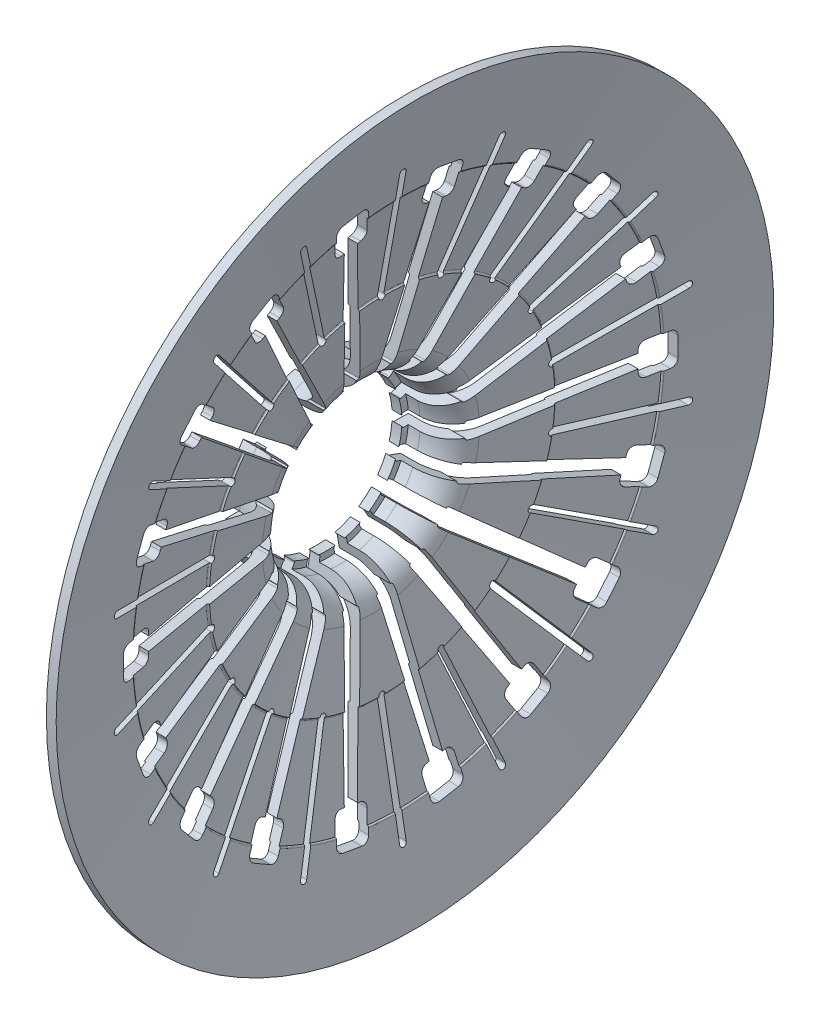
SolidWorks part; units mm, degrees
ref_plane "Front Plane" through (0, 0, 0) normal (0, 0, 1) x (1, 0, 0)
ref_plane "Top Plane" through (0, 0, 0) normal (0, 1, 0) x (1, 0, 0)
ref_plane "Right Plane" through (0, 0, 0) normal (1, 0, 0) x (0, 0, -1)
other "Configuration Table"
sketch "Sketch2" plane through (0, 0, 0) normal (0, 0, 1) x (1, 0, 0)
  line L0 (1418.6702, 525.6363) -> (1415.6702, 525.6363)
  line L1 (1418.6702, 415.6363) -> (1388.6702, 415.6363) construction
  line L2 (1388.6702, 415.6363) -> (1388.6702, 443.6363)
  line L3 (1415.6702, 525.6363) -> (1410.6453, 497.1385)
  line L4 (1418.6702, 415.6363) -> (1418.6702, 525.6363) construction
  line L5 (1388.6702, 443.6363) -> (1392.8204, 443.6363)
  line L6 (1418.6702, 525.6363) -> (1413.6453, 497.1385)
  line L7 (1325.0417, 415.6363) -> (1423.6069, 415.6363) construction
  line L8 (1388.6702, 415.6363) -> (1391.6702, 415.6363)
  line L9 (1391.6702, 440.6363) -> (1395.2915, 440.6363)
  line L10 (1391.6702, 415.6363) -> (1391.6702, 440.6363)
  line L11 (1410.1533, 496.7273) -> (1405.181, 469.169)
  line L12 (1408.6104, 468.5841) -> (1405.1395, 448.8998)
  line L13 (1405.6104, 468.5841) -> (1402.6685, 451.8998)
  line L30 (1413.1533, 496.7273) -> (1408.181, 469.169)
  arc A0 (1392.8204, 443.6363) -> (1402.6685, 451.8998) centre (1392.8204, 453.6363) ccw
  arc A1 (1395.2915, 440.6363) -> (1405.1395, 448.8998) centre (1395.2915, 450.6363) ccw
  arc A10 (1413.1533, 496.7273) -> (1413.6453, 497.1385) centre (1413.1533, 497.2273) ccw
  arc A11 (1405.181, 469.169) -> (1405.6104, 468.5841) centre (1405.6731, 469.0802) ccw
  arc A12 (1408.181, 469.169) -> (1408.6104, 468.5841) centre (1408.6731, 469.0802) ccw
  arc A13 (1410.1533, 496.7273) -> (1410.6453, 497.1385) centre (1410.1533, 497.2273) ccw
  dimension "D5" = 10
  dimension "D6" = 10
  dimension "D2" = 30
  dimension "D3" = 110
  dimension "D4" = 3
revolve "Revolve1" add sketch "Sketch2" angle 360 about L7
sketch "Sketch8" plane through (0, 0, 0) normal (1, 0, 0) x (0, 0, -1)
  line L0 (0, 525.6363) -> (0, 504.6363) construction
  line L1 (0, 504.6363) -> (0, 468.6363) construction
  line L2 (30.4398, 499.269) -> (18.1271, 465.44) construction
  line L3 (1, 504.6363) -> (1, 468.6363)
  line L4 (-1, 504.6363) -> (-1, 468.6363)
  line L5 (31.3795, 498.9269) -> (19.0668, 465.098)
  line L6 (29.5001, 499.611) -> (17.1874, 465.7821)
  line L7 (57.2081, 483.8143) -> (34.0677, 456.2367) construction
  line L8 (57.9741, 483.1715) -> (34.8338, 455.5939)
  line L9 (56.4421, 484.4571) -> (33.3017, 456.8795)
  line L10 (77.0763, 460.1363) -> (45.8993, 442.1363) construction
  line L11 (77.5763, 459.2703) -> (46.3993, 441.2703)
  line L12 (76.5763, 461.0023) -> (45.3993, 443.0023)
  line L13 (87.6479, 431.091) -> (52.1948, 424.8397) construction
  line L14 (87.8215, 430.1062) -> (52.3685, 423.8549)
  line L15 (87.4742, 432.0758) -> (52.0212, 425.8245)
  line L16 (87.6479, 400.1816) -> (52.1948, 406.433) construction
  line L17 (87.4742, 399.1968) -> (52.0212, 405.4482)
  line L18 (87.8215, 401.1664) -> (52.3685, 407.4178)
  line L19 (77.0763, 371.1363) -> (45.8993, 389.1363) construction
  line L20 (76.5763, 370.2703) -> (45.3993, 388.2703)
  line L21 (77.5763, 372.0023) -> (46.3993, 390.0023)
  line L22 (57.2081, 347.4584) -> (34.0677, 375.036) construction
  line L23 (56.4421, 346.8156) -> (33.3017, 374.3932)
  line L24 (57.9741, 348.1012) -> (34.8338, 375.6788)
  line L25 (30.4398, 332.0037) -> (18.1271, 365.8326) construction
  line L26 (29.5001, 331.6617) -> (17.1874, 365.4906)
  line L27 (31.3795, 332.3457) -> (19.0668, 366.1746)
  line L28 (0, 326.6363) -> (0, 362.6363) construction
  line L29 (-1, 326.6363) -> (-1, 362.6363)
  line L30 (1, 326.6363) -> (1, 362.6363)
  line L31 (-30.4398, 332.0037) -> (-18.1271, 365.8326) construction
  line L32 (-31.3795, 332.3457) -> (-19.0668, 366.1746)
  line L33 (-29.5001, 331.6617) -> (-17.1874, 365.4906)
  line L34 (-57.2081, 347.4584) -> (-34.0677, 375.036) construction
  line L35 (-57.9741, 348.1012) -> (-34.8338, 375.6788)
  line L36 (-56.4421, 346.8156) -> (-33.3017, 374.3932)
  line L37 (-77.0763, 371.1363) -> (-45.8993, 389.1363) construction
  line L38 (-77.5763, 372.0023) -> (-46.3993, 390.0023)
  line L39 (-76.5763, 370.2703) -> (-45.3993, 388.2703)
  line L40 (-87.6479, 400.1816) -> (-52.1948, 406.433) construction
  line L41 (-87.8215, 401.1664) -> (-52.3685, 407.4178)
  line L42 (-87.4742, 399.1968) -> (-52.0212, 405.4482)
  line L43 (-87.6479, 431.091) -> (-52.1948, 424.8397) construction
  line L44 (-87.4742, 432.0758) -> (-52.0212, 425.8245)
  line L45 (-87.8215, 430.1062) -> (-52.3685, 423.8549)
  line L46 (-77.0763, 460.1363) -> (-45.8993, 442.1363) construction
  line L47 (-76.5763, 461.0023) -> (-45.3993, 443.0023)
  line L48 (-77.5763, 459.2703) -> (-46.3993, 441.2703)
  line L49 (-57.2081, 483.8143) -> (-34.0677, 456.2367) construction
  line L50 (-56.4421, 484.4571) -> (-33.3017, 456.8795)
  line L51 (-57.9741, 483.1715) -> (-34.8338, 455.5939)
  line L52 (-30.4398, 499.269) -> (-18.1271, 465.44) construction
  line L53 (-29.5001, 499.611) -> (-17.1874, 465.7821)
  line L54 (-31.3795, 498.9269) -> (-19.0668, 465.098)
  circle A0 centre (0, 415.6363) radius 110 construction
  arc A1 (1, 504.6363) -> (-1, 504.6363) centre (0, 504.6363) ccw
  arc A2 (-1, 468.6363) -> (1, 468.6363) centre (0, 468.6363) ccw
  arc A3 (31.3795, 498.9269) -> (29.5001, 499.611) centre (30.4398, 499.269) ccw
  arc A4 (17.1874, 465.7821) -> (19.0668, 465.098) centre (18.1271, 465.44) ccw
  arc A5 (57.9741, 483.1715) -> (56.4421, 484.4571) centre (57.2081, 483.8143) ccw
  arc A6 (33.3017, 456.8795) -> (34.8338, 455.5939) centre (34.0677, 456.2367) ccw
  arc A7 (77.5763, 459.2703) -> (76.5763, 461.0023) centre (77.0763, 460.1363) ccw
  arc A8 (45.3993, 443.0023) -> (46.3993, 441.2703) centre (45.8993, 442.1363) ccw
  arc A9 (87.8215, 430.1062) -> (87.4742, 432.0758) centre (87.6479, 431.091) ccw
  arc A10 (52.0212, 425.8245) -> (52.3685, 423.8549) centre (52.1948, 424.8397) ccw
  arc A11 (87.4742, 399.1968) -> (87.8215, 401.1664) centre (87.6479, 400.1816) ccw
  arc A12 (52.3685, 407.4178) -> (52.0212, 405.4482) centre (52.1948, 406.433) ccw
  arc A13 (76.5763, 370.2703) -> (77.5763, 372.0023) centre (77.0763, 371.1363) ccw
  arc A14 (46.3993, 390.0023) -> (45.3993, 388.2703) centre (45.8993, 389.1363) ccw
  arc A15 (56.4421, 346.8156) -> (57.9741, 348.1012) centre (57.2081, 347.4584) ccw
  arc A16 (34.8338, 375.6788) -> (33.3017, 374.3932) centre (34.0677, 375.036) ccw
  arc A17 (29.5001, 331.6617) -> (31.3795, 332.3457) centre (30.4398, 332.0037) ccw
  arc A18 (19.0668, 366.1746) -> (17.1874, 365.4906) centre (18.1271, 365.8326) ccw
  arc A19 (-1, 326.6363) -> (1, 326.6363) centre (0, 326.6363) ccw
  arc A20 (1, 362.6363) -> (-1, 362.6363) centre (0, 362.6363) ccw
  arc A21 (-31.3795, 332.3457) -> (-29.5001, 331.6617) centre (-30.4398, 332.0037) ccw
  arc A22 (-17.1874, 365.4906) -> (-19.0668, 366.1746) centre (-18.1271, 365.8326) ccw
  arc A23 (-57.9741, 348.1012) -> (-56.4421, 346.8156) centre (-57.2081, 347.4584) ccw
  arc A24 (-33.3017, 374.3932) -> (-34.8338, 375.6788) centre (-34.0677, 375.036) ccw
  arc A25 (-77.5763, 372.0023) -> (-76.5763, 370.2703) centre (-77.0763, 371.1363) ccw
  arc A26 (-45.3993, 388.2703) -> (-46.3993, 390.0023) centre (-45.8993, 389.1363) ccw
  arc A27 (-87.8215, 401.1664) -> (-87.4742, 399.1968) centre (-87.6479, 400.1816) ccw
  arc A28 (-52.0212, 405.4482) -> (-52.3685, 407.4178) centre (-52.1948, 406.433) ccw
  arc A29 (-87.4742, 432.0758) -> (-87.8215, 430.1062) centre (-87.6479, 431.091) ccw
  arc A30 (-52.3685, 423.8549) -> (-52.0212, 425.8245) centre (-52.1948, 424.8397) ccw
  arc A31 (-76.5763, 461.0023) -> (-77.5763, 459.2703) centre (-77.0763, 460.1363) ccw
  arc A32 (-46.3993, 441.2703) -> (-45.3993, 443.0023) centre (-45.8993, 442.1363) ccw
  arc A33 (-56.4421, 484.4571) -> (-57.9741, 483.1715) centre (-57.2081, 483.8143) ccw
  arc A34 (-34.8338, 455.5939) -> (-33.3017, 456.8795) centre (-34.0677, 456.2367) ccw
  arc A35 (-29.5001, 499.611) -> (-31.3795, 498.9269) centre (-30.4398, 499.269) ccw
  arc A36 (-19.0668, 465.098) -> (-17.1874, 465.7821) centre (-18.1271, 465.44) ccw
  point P9 (0, 486.6363)
  point P17 (24.2834, 482.3545)
  point P24 (45.6379, 470.0255)
  point P31 (61.4878, 451.1363)
  point P38 (69.9214, 427.9653)
  point P45 (69.9214, 403.3073)
  point P52 (61.4878, 380.1363)
  point P59 (45.6379, 361.2472)
  point P66 (24.2834, 348.9181)
  point P73 (0, 344.6363)
  point P80 (-24.2834, 348.9181)
  point P87 (-45.6379, 361.2472)
  point P94 (-61.4878, 380.1363)
  point P101 (-69.9214, 403.3073)
  point P108 (-69.9214, 427.9653)
  point P115 (-61.4878, 451.1363)
  point P122 (-45.6379, 470.0255)
  point P129 (-24.2834, 482.3545)
  point P134 (0, 415.6363)
  dimension "D1" = 18
extrude "Cut-Extrude3" cut sketch "Sketch8" along normal blind 1469.5
sketch "Sketch9" plane through (1388.6702, 0, 0) normal (-1, 0, 0) x (0, 0, 1)
  line L0 (-7.2421, 444.8221) -> (-7.1791, 444.8333)
  line L1 (-3.1768, 445.539) -> (-3.2398, 445.5279)
  line L6 (-17.7214, 498.8356) -> (-14.767, 499.3565)
  line L7 (-15.0632, 489.15) -> (-15.985, 488.9875)
  line L8 (-18.3019, 490.6098) -> (-19.3438, 496.5186)
  line L9 (-10.0761, 490.0294) -> (-10.9932, 489.8677)
  line L10 (-8.4538, 492.3463) -> (-9.4957, 498.2551)
  line L11 (-2.1028, 439.0794) -> (-3.2398, 445.5279)
  line L12 (-6.042, 438.3848) -> (-7.1791, 444.8333)
  line L19 (-10.9932, 489.8677) -> (-2.7712, 446.1182)
  line L20 (-15.0632, 489.15) -> (-7.8213, 445.2277)
  line L21 (-11.8126, 499.8774) -> (-14.767, 499.3565)
  arc A0 (-2.54, 438.4956) -> (-5.4315, 437.9858) centre (0, 415.6363) ccw
  arc A4 (-17.7214, 498.8356) -> (-19.3438, 496.5186) centre (-17.3741, 496.8659) ccw
  arc A5 (-18.3019, 490.6098) -> (-15.985, 488.9875) centre (-16.3323, 490.9571) ccw
  arc A6 (-9.4957, 498.2551) -> (-11.8126, 499.8774) centre (-11.4653, 497.9078) ccw
  arc A7 (-10.0761, 490.0294) -> (-8.4538, 492.3463) centre (-10.4234, 491.999) ccw
  arc A8 (-2.54, 438.4956) -> (-2.1028, 439.0794) centre (-2.5952, 438.9926) ccw
  arc A9 (-6.042, 438.3848) -> (-5.4315, 437.9858) centre (-5.5496, 438.4716) ccw
  arc A10 (-3.1768, 445.539) -> (-2.7712, 446.1182) centre (-3.2636, 446.0314) ccw
  arc A11 (-7.8213, 445.2277) -> (-7.2421, 444.8221) centre (-7.3289, 445.3145) ccw
extrude "Cut-Extrude4" cut sketch "Sketch9" against normal through all
sketch "Sketch10" plane through (1388.6702, 0, 0) normal (-1, 0, 0) x (0, 0, 1)
  circle A0 centre (0, 415.6363) radius 23
extrude "Cut-Extrude5" cut sketch "Sketch10" against normal through all
pattern_circular "CirPattern3" count 18 over 360 about axis through (0, 415.6363, 0) along (1, 0, 0) of "Cut-Extrude4"
